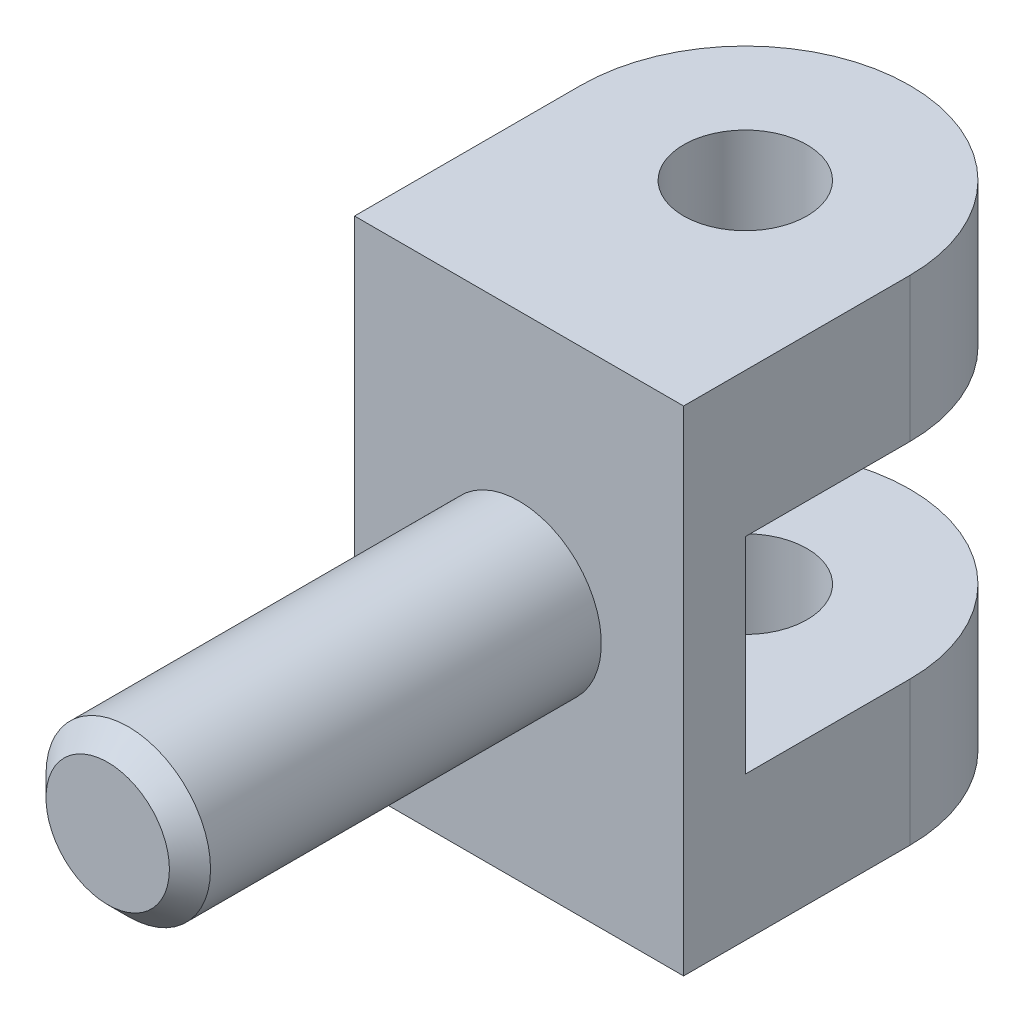
from build123d import *

# Parameters (mm, degrees)
BOSS_EXTRUDE1_DEPTH = 12
SKETCH2_R           = 4
BOSS_EXTRUDE2_DEPTH = 20
SKETCH3_W           = 32
SKETCH3_H           = 10
CUT_EXTRUDE1_DEPTH  = 20
SKETCH4_R           = 3
CUT_EXTRUDE2_DEPTH  = 34
CHAMFER1_SIZE       = 1


with BuildPart() as part:
    # Sketch1 → Boss-Extrude1 (new, symmetric)
    with BuildSketch(Plane(origin=(0, 0, 0), x_dir=(1, 0, 0), z_dir=(0, 1, 0))):
        with BuildLine():
            Line((-8, 0), (-8, -11))
            Line((-8, -11), (8, -11))
            Line((8, -11), (8, 0))
            ThreePointArc((8, 0), (0, 8), (-8, 0))
        make_face()
    extrude(amount=BOSS_EXTRUDE1_DEPTH, both=True)

    # Sketch2 → Boss-Extrude2 (add)
    with BuildSketch(Plane.XY.offset(11)):
        with Locations(Location((0, 0, 0), (0, 0, 180))):
            Circle(SKETCH2_R)
    extrude(amount=BOSS_EXTRUDE2_DEPTH)

    # Sketch3 → Cut-Extrude1 (cut)
    with BuildSketch(Plane(origin=(8, 0, 0), x_dir=(0, 0, -1), z_dir=(1, 0, 0))):
        with Locations((8, 0)):
            Rectangle(SKETCH3_W, SKETCH3_H)
    extrude(amount=-CUT_EXTRUDE1_DEPTH, mode=Mode.SUBTRACT)

    # Sketch4 → Cut-Extrude2 (cut)
    with BuildSketch(Plane.XZ.offset(12)):
        with Locations(Location((0, 0, 0), (0, 0, 270))):
            Circle(SKETCH4_R)
    extrude(amount=-CUT_EXTRUDE2_DEPTH, mode=Mode.SUBTRACT)

    # Chamfer1
    chamfer1_edges = [part.edges().sort_by_distance(p)[0] for p in [
        (4, 0, 31),
    ]]
    chamfer(chamfer1_edges, length=CHAMFER1_SIZE)


solid = part.part
